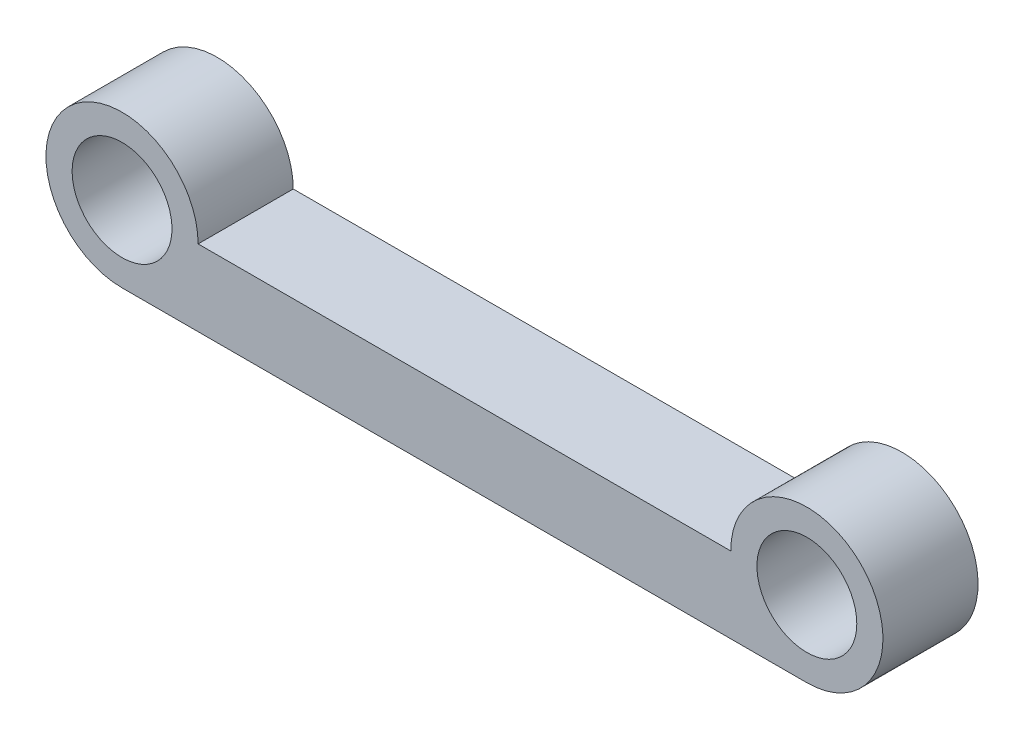
from build123d import *

# Parameters (mm, degrees)
SKETCH1_W            = 35
SKETCH1_H            = 5
BOSS_EXTRUDE3_DEPTH  = 5
SKETCH7_W            = 5
SKETCH7_H            = 5
BOSS_EXTRUDE6_DEPTH  = 5
FILLET6_R            = 1
FILLET7_R            = 1
SKETCH11_R           = 2
CUT_EXTRUDE2_DEPTH   = 5
SKETCH5_R            = 2.375
BOSS_EXTRUDE9_DEPTH  = 5
SKETCH13_R           = 4
BOSS_EXTRUDE10_DEPTH = 5
SKETCH14_R           = 2.625
CUT_EXTRUDE3_DEPTH   = 25.84321589
SKETCH15_W           = 5
SKETCH15_H           = 5
BOSS_EXTRUDE11_DEPTH = 0.875
FILLET8_R            = 2
FILLET9_R            = 2
SKETCH16_R           = 4
BOSS_EXTRUDE12_DEPTH = 5
SKETCH17_R           = 2.625
CUT_EXTRUDE4_DEPTH   = 30
CUT_EXTRUDE5_DEPTH   = 25.84321589
BOSS_EXTRUDE13_DEPTH = 5


with BuildPart() as part:
    # Sketch1 → Boss-Extrude3 (new body)
    with BuildSketch(Plane.XY):
        Rectangle(SKETCH1_W, SKETCH1_H)
    extrude(amount=BOSS_EXTRUDE3_DEPTH)

    # Sketch7 → Boss-Extrude6 (add)
    with BuildSketch(Plane.XY.offset(5)):
        with Locations((20, 0.046210476)):
            Rectangle(SKETCH7_W, SKETCH7_H)
    extrude(amount=-BOSS_EXTRUDE6_DEPTH)

    # Fillet6
    fillet6_edges = [part.edges().sort_by_distance(p)[0] for p in [
        (22.5, 2.546210476, 2.5),
    ]]
    fillet(fillet6_edges, radius=FILLET6_R)

    # Fillet7
    fillet7_edges = [part.edges().sort_by_distance(p)[0] for p in [
        (22.5, -2.453789524, 2.5),
    ]]
    fillet(fillet7_edges, radius=FILLET7_R)

    # Sketch11 → Cut-Extrude2 (cut)
    with BuildSketch(Plane.XY.offset(5)):
        with Locations((20, 0.023105238)):
            Circle(SKETCH11_R)
    extrude(amount=-CUT_EXTRUDE2_DEPTH, mode=Mode.SUBTRACT)

    # Sketch5 → Boss-Extrude9 (add)
    with BuildSketch(Plane.XY.offset(5)):
        with Locations(Location((-16, 0, 0), (0, 0, 230.833289284))):
            Circle(SKETCH5_R)
    extrude(amount=BOSS_EXTRUDE9_DEPTH)

    # Sketch13 → Boss-Extrude10 (add, through all)
    with BuildSketch(Plane.XY.offset(5)):
        with Locations((20, 0.023105238)):
            Circle(SKETCH13_R)
    extrude(amount=-BOSS_EXTRUDE10_DEPTH)

    # Sketch14 → Cut-Extrude3 (cut, through all)
    with BuildSketch(Plane.XY.offset(5)):
        with Locations((20, 0.023105238)):
            Circle(SKETCH14_R)
    extrude(amount=-CUT_EXTRUDE3_DEPTH, mode=Mode.SUBTRACT)

    # Sketch15 → Boss-Extrude11 (add, through all)
    with BuildSketch(Plane.ZY.offset(17.5)):
        with Locations((2.5, 0)):
            Rectangle(SKETCH15_W, SKETCH15_H)
    extrude(amount=BOSS_EXTRUDE11_DEPTH)

    # Fillet8
    fillet8_edges = [part.edges().sort_by_distance(p)[0] for p in [
        (-18.375, 2.5, 2.5),
    ]]
    fillet(fillet8_edges, radius=FILLET8_R)

    # Fillet9
    fillet9_edges = [part.edges().sort_by_distance(p)[0] for p in [
        (-18.375, -2.5, 2.5),
    ]]
    fillet(fillet9_edges, radius=FILLET9_R)

    # Sketch16 → Boss-Extrude12 (add)
    with BuildSketch(Plane.XY.offset(5)):
        with Locations((-16, 0)):
            Circle(SKETCH16_R)
    extrude(amount=-BOSS_EXTRUDE12_DEPTH)

    # Sketch17 → Cut-Extrude4 (cut)
    with BuildSketch(Plane.XY.offset(10)):
        with Locations(Location((-16, 0, 0), (0, 0, 180))):
            Circle(SKETCH17_R)
    extrude(amount=-CUT_EXTRUDE4_DEPTH, mode=Mode.SUBTRACT)

    # Sketch18 → Cut-Extrude5 (cut, through all)
    with BuildSketch(Plane.XY.offset(5)):
        with BuildLine():
            Line((-12, 0), (16, 0.023105238))
            ThreePointArc((16, 0.023105238), (17.170665329, 2.850624525), (19.99743266, 4.023104414))
            Line((19.99743266, 4.023104414), (-16, 4))
            ThreePointArc((-16, 4), (-13.171572875, 2.828427125), (-12, 0))
        make_face()
    extrude(amount=-CUT_EXTRUDE5_DEPTH, mode=Mode.SUBTRACT)

    # Sketch19 → Boss-Extrude13 (add, through all)
    with BuildSketch(Plane.XY.offset(5)):
        Polygon((-16, -4), (20, -3.976894762), (16, -1.273335264), (-12.878635235, -1.649219819), align=None)
    extrude(amount=-BOSS_EXTRUDE13_DEPTH)


solid = part.part
